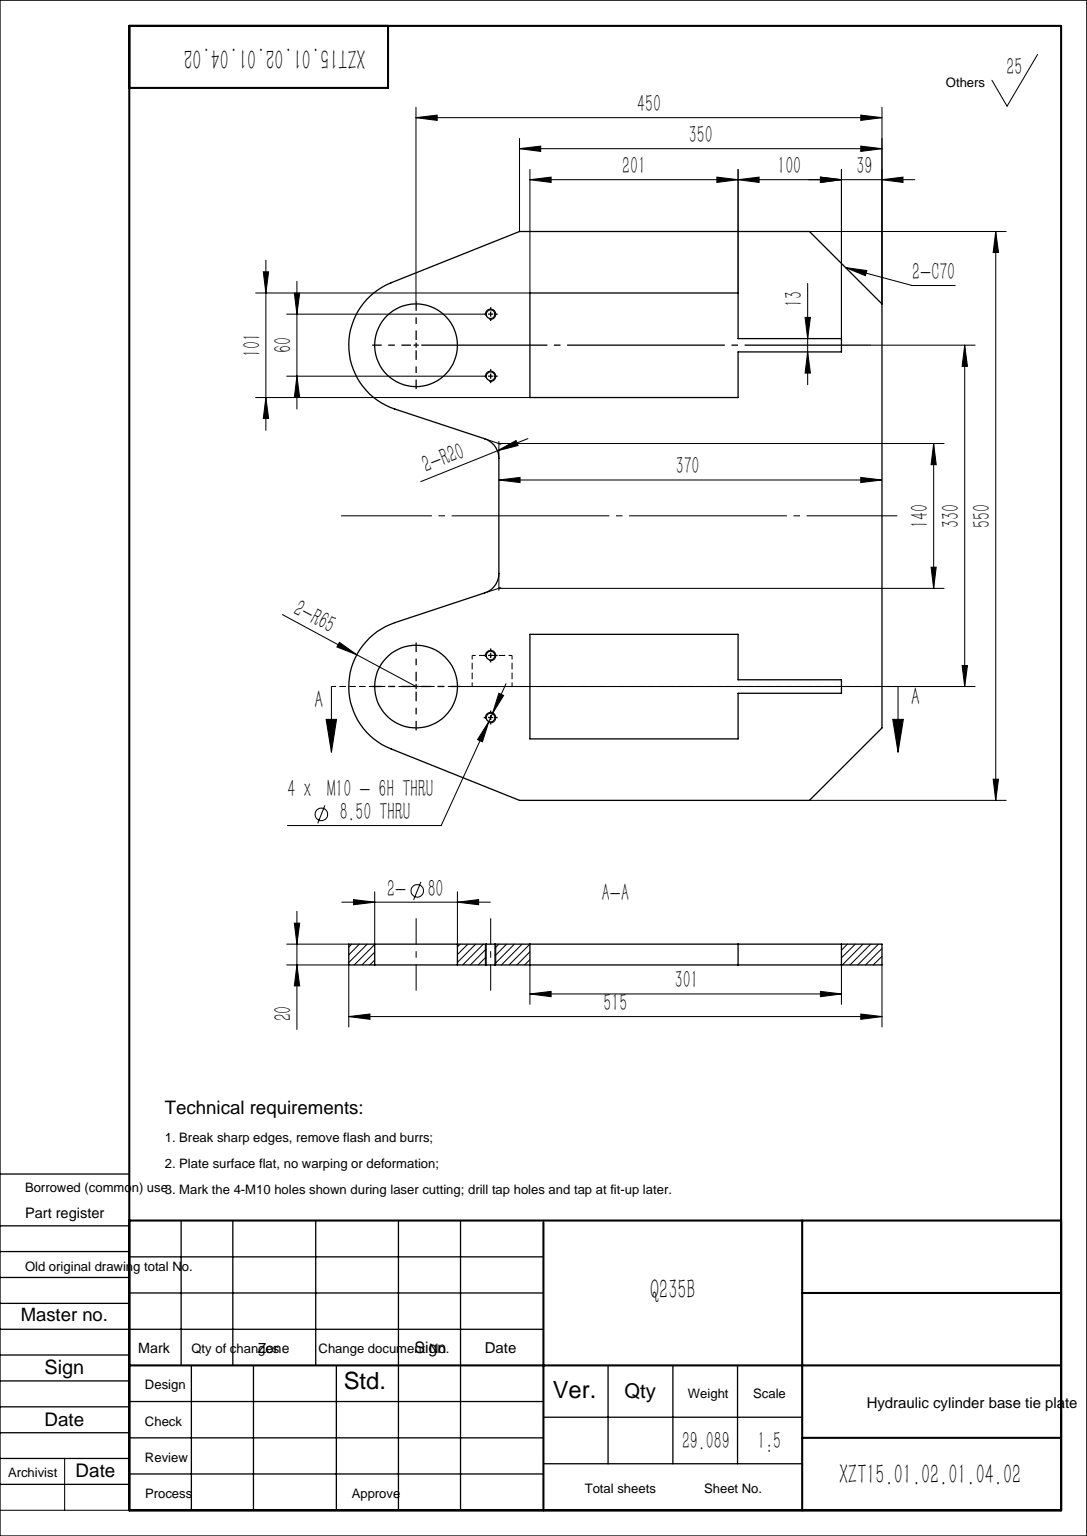
SolidWorks part; units mm, degrees
material "Q235B"
ref_plane "Front Plane" through (0, 0, 0) normal (0, 0, 1) x (1, 0, 0)
ref_plane "Top Plane" through (0, 0, 0) normal (0, 1, 0) x (1, 0, 0)
ref_plane "Right Plane" through (0, 0, 0) normal (1, 0, 0) x (0, 0, -1)
sketch "Sketch1" plane through (0, 0, 0) normal (0, 0, 1) x (1, 0, 0)
  line L0 (0, -70) -> (0, 70)
  line L1 (0, 70) -> (-100.4538, 103.302)
  line L2 (-104.1374, 225.3522) -> (20, 275)
  line L3 (20, 275) -> (370, 275)
  line L4 (370, 275) -> (370, -275)
  line L5 (370, 0) -> (0, 0) construction
  line L6 (20, -275) -> (370, -275)
  line L7 (-104.1374, -225.3522) -> (20, -275)
  line L8 (0, -70) -> (-100.4538, -103.302)
  line L9 (231, 158.5) -> (231, 114.5)
  line L10 (30, 215.5) -> (231, 215.5)
  line L11 (30, 215.5) -> (30, 114.5)
  line L12 (30, 114.5) -> (231, 114.5)
  line L13 (231, 215.5) -> (231, 171.5)
  line L14 (231, 171.5) -> (331, 171.5)
  line L16 (231, 158.5) -> (331, 158.5)
  line L17 (331, 171.5) -> (331, 158.5)
  line L18 (-80, 165) -> (30, 165) construction
  line L19 (-80, -165) -> (30, -165) construction
  line L20 (331, -171.5) -> (331, -158.5)
  line L21 (231, -158.5) -> (331, -158.5)
  line L22 (231, -171.5) -> (331, -171.5)
  line L23 (231, -215.5) -> (231, -171.5)
  line L24 (30, -114.5) -> (231, -114.5)
  line L25 (30, -215.5) -> (30, -114.5)
  line L26 (30, -215.5) -> (231, -215.5)
  line L27 (231, -158.5) -> (231, -114.5)
  arc A0 (-100.4538, 103.302) -> (-104.1374, 225.3522) centre (-80, 165) cw
  arc A1 (-100.4538, -103.302) -> (-104.1374, -225.3522) centre (-80, -165) ccw
  circle A2 centre (-80, 165) radius 40
  circle A3 centre (-80, -165) radius 40
  point P24 (30, 165)
  dimension "D1" = 65
  dimension "D2" = 80
  dimension "D3" = 101
  dimension "D4" = 201
  dimension "D5" = 100
  dimension "D6" = 39
  dimension "D7" = 13
  dimension "D8" = 6.5
  dimension "D9" = 330
  dimension "D10" = 550
  dimension "D11" = 450
  dimension "D12" = 350
  dimension "D13" = 140
  dimension "D14" = 370
extrude "Boss-Extrude1" add sketch "Sketch1" along normal blind 20
hole_wizard "M10 Tapped Hole1" positions "Sketch2" profile "Sketch3" tap size "M10" standard "GB" end condition up to next
sketch "Sketch2" plane through (0, 0, 20) normal (0, 0, 1) x (1, 0, 0)
  line L0 (-80, 165) -> (38.1087, 165) construction
  line L2 (370, -275) -> (370, 275) construction
  line L3 (0, 0) -> (-155.2888, 0) construction
  point P0 (-8, 195)
  point P7 (-8, 135)
  point P14 (-8, -135)
  point P15 (-8, -195)
  dimension "D1" = 60
  dimension "D2" = 378
sketch "Sketch3" plane through (-8, 195, 20) normal (1, 0, 0) x (0, -1, 0)
  line L0 (0, 0) -> (0, 20)
  line L1 (0, 20) -> (4.25, 20)
  line L2 (4.25, 20) -> (4.25, 0)
  line L5 (4.25, 0) -> (0, 0)
  line L11 (0, -6.35) -> (0, 107.95) construction
  dimension "通孔螺纹孔钻头直径" = 8.5
  dimension "通孔螺纹孔钻头深度" = 20
cosmetic thread "Cosmetic Thread 1" parameters "D2"=10
cosmetic thread "Cosmetic Thread 2" parameters "D2"=10
cosmetic thread "Cosmetic Thread 3" parameters "D2"=10
cosmetic thread "Cosmetic Thread 4" parameters "D2"=10
chamfer "Chamfer1" distance 70 angle 45 2 edges at (370, -275, 10) (370, 275, 10)
fillet "Fillet1" radius 20 2 edges at (0, -70, 10) (0, 70, 10)
